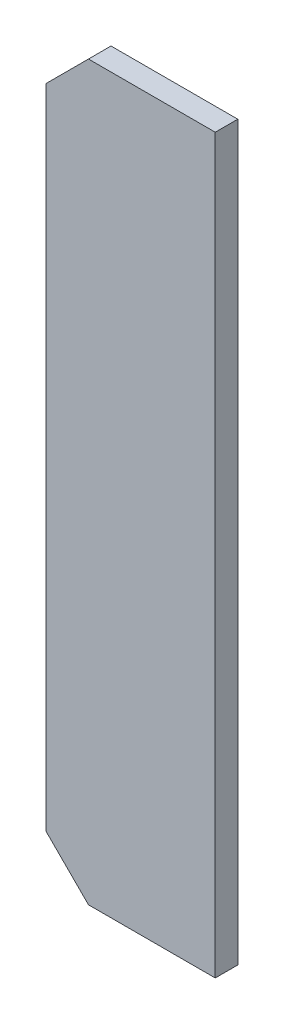
SolidWorks part; units mm, degrees
material "Q235B"
ref_plane "Front Plane" through (0, 0, 0) normal (0, 0, 1) x (1, 0, 0)
ref_plane "Top Plane" through (0, 0, 0) normal (0, 1, 0) x (1, 0, 0)
ref_plane "Right Plane" through (0, 0, 0) normal (1, 0, 0) x (0, 0, -1)
sketch "Sketch1" plane through (0, 0, 0) normal (0, 0, 1) x (1, 0, 0)
  line L1 (30, -130) -> (-30, -130)
  line L2 (30, -130) -> (30, 130)
  line L3 (30, 130) -> (-30, 130)
  line L4 (-30, -130) -> (-30, 130)
  line L5 (30, -130) -> (-30, 130) construction
  line L6 (30, 130) -> (-30, -130) construction
  point P0 (0, 0)
  dimension "D1" = 260
  dimension "D2" = 60
extrude "Boss-Extrude1" add sketch "Sketch1" along normal blind 8
chamfer "Chamfer1" distance 15 angle 45 2 edges at (-30, -130, 4) (-30, 130, 4)
